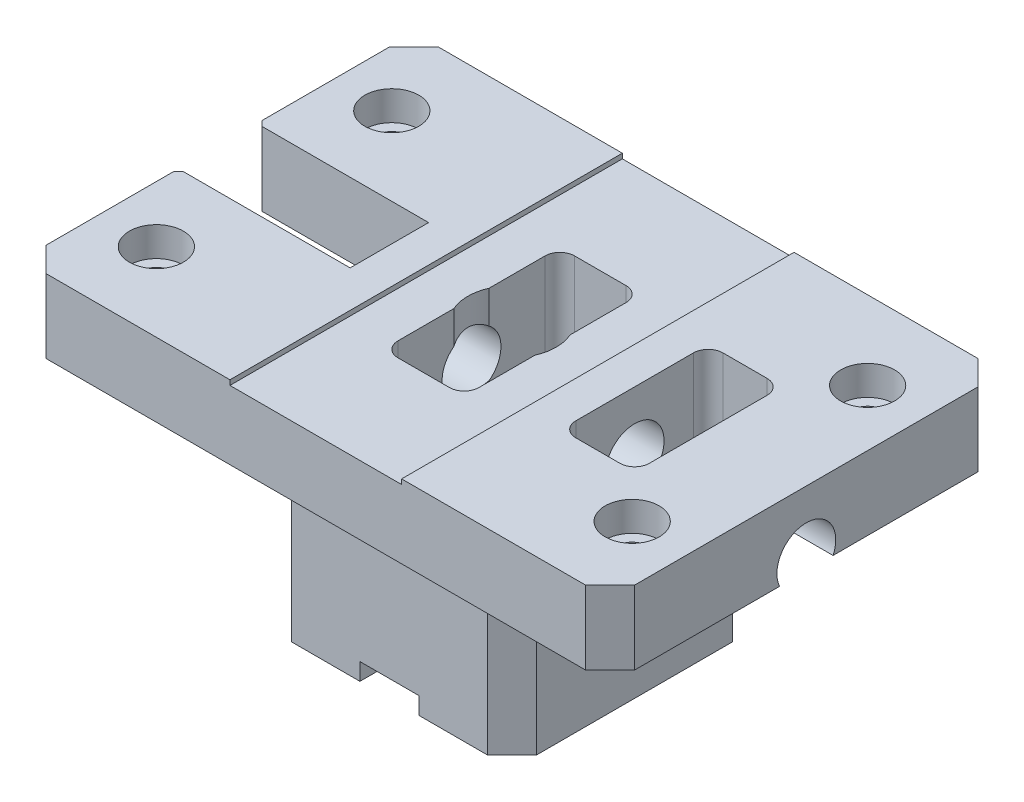
SolidWorks part; units mm, degrees
ref_plane "Front Plane" through (0, 0, 0) normal (0, 0, 1) x (1, 0, 0)
ref_plane "Top Plane" through (0, 0, 0) normal (0, 1, 0) x (1, 0, 0)
ref_plane "Right Plane" through (0, 0, 0) normal (1, 0, 0) x (0, 0, -1)
sketch "Sketch1" plane through (0, 0, 0) normal (0, 1, 0) x (1, 0, 0)
  line L1 (-60, 40) -> (60, 40)
  line L2 (-60, 40) -> (-60, -40)
  line L3 (-60, -40) -> (60, -40)
  line L4 (60, 40) -> (60, -40)
  line L5 (-60, 40) -> (60, -40) construction
  line L6 (-60, -40) -> (60, 40) construction
  point P0 (0, 0)
  dimension "D1" = 120
  dimension "D2" = 80
extrude "Boss-Extrude1" add sketch "Sketch1" along normal blind 15
sketch "Sketch2" plane through (0, 0, 0) normal (0, -1, 0) x (1, 0, 0)
  line L1 (-25, 25) -> (25, 25)
  line L2 (-25, 25) -> (-25, -25)
  line L3 (-25, -25) -> (25, -25)
  line L4 (25, 25) -> (25, -25)
  line L5 (-25, 25) -> (25, -25) construction
  line L6 (-25, -25) -> (25, 25) construction
  point P0 (0, 0)
  dimension "D1" = 50
  dimension "D2" = 50
extrude "Boss-Extrude2" add sketch "Sketch2" along normal blind 40
sketch "Sketch4" plane through (0, 15, 0) normal (0, 1, 0) x (1, 0, 0)
  line L1 (-5.25, 18) -> (5.25, 18)
  line L2 (-8.25, 15) -> (-8.25, -15)
  line L3 (-5.25, -18) -> (5.25, -18)
  line L4 (8.25, 15) -> (8.25, -15)
  line L5 (-8.25, 18) -> (8.25, -18) construction
  line L6 (-8.25, -18) -> (8.25, 18) construction
  arc A0 (-8.25, -15) -> (-5.25, -18) centre (-5.25, -15) ccw
  arc A1 (5.25, -18) -> (8.25, -15) centre (5.25, -15) ccw
  arc A2 (5.25, 18) -> (8.25, 15) centre (5.25, 15) cw
  arc A3 (-5.25, 18) -> (-8.25, 15) centre (-5.25, 15) ccw
  point P0 (0, 0)
  dimension "D3" = 3
  dimension "D1" = 16.5
  dimension "D2" = 36
extrude "Cut-Extrude2" cut sketch "Sketch4" against normal blind 33
sketch "Sketch5" plane through (-60, 0, 0) normal (-1, 0, 0) x (0, 0, 1)
  line L1 (-8, 20.6201) -> (8, 20.6201)
  line L2 (-8, 20.6201) -> (-8, -20.6201)
  line L3 (-8, -20.6201) -> (8, -20.6201)
  line L4 (8, 20.6201) -> (8, -20.6201)
  line L5 (-8, 20.6201) -> (8, -20.6201) construction
  line L6 (-8, -20.6201) -> (8, 20.6201) construction
  point P0 (0, 0)
  dimension "D1" = 16
  dimension "D2" = 41.2401
extrude "Cut-Extrude3" cut sketch "Sketch5" against normal blind 35
sketch "Sketch6" plane through (-25, 0, 0) normal (-1, 0, 0) x (0, 0, 1)
  line L0 (-8, 15) -> (8, 15) construction
  circle A0 centre (0, 2.5) radius 6
  dimension "D1" = 12
  dimension "D2" = 12.5
extrude "Cut-Extrude4" cut sketch "Sketch6" against normal through all
hole_wizard "CBORE for M6 Hex Socket Head Cap Screw1" positions "Sketch10" profile "Sketch9" counterbore size "M6" standard "ISO" end condition through all
sketch "Sketch10" plane through (0, 15, 0) normal (0, 1, 0) x (-1, 0, 0)
  line L0 (0, -40) -> (0, 40) construction
  line L1 (-60, -40) -> (60, -40) construction
  line L2 (60, 40) -> (-60, 40) construction
  line L4 (25, 0) -> (-31.5815, 0) construction
  line L5 (25, -8) -> (25, 8) construction
  point P1 (48.5, 24)
  point P3 (-48.5, 24)
  point P5 (-48.5, -24)
  point P7 (48.5, -24)
  dimension "D1" = 48
  dimension "D2" = 97
sketch "Sketch9" plane through (-48.5, 15, 24) normal (1, 0, 0) x (0, 0, 1)
  line L0 (0, 0) -> (0, 55)
  line L1 (0, 55) -> (3.3, 55)
  line L3 (3.3, 55) -> (3.3, 6)
  line L4 (3.3, 6) -> (5.5, 6)
  line L5 (5.5, 6) -> (5.5, 0)
  line L7 (5.5, 0) -> (0, 0)
  line L11 (0, -6.35) -> (0, 107.95) construction
  dimension "通孔孔直径" = 6.6
  dimension "通孔孔深度" = 55
  dimension "柱形沉头孔直径" = 11
  dimension "柱形沉头孔深度" = 6
sketch "Sketch11" plane through (0, -40, 0) normal (0, -1, 0) x (1, 0, 0)
  line L1 (-6, 30) -> (6, 30)
  line L2 (-6, 30) -> (-6, -30)
  line L3 (-6, -30) -> (6, -30)
  line L4 (6, 30) -> (6, -30)
  line L5 (-6, 30) -> (6, -30) construction
  line L6 (-6, -30) -> (6, 30) construction
  point P0 (0, 0)
  dimension "D1" = 12
  dimension "D2" = 60
extrude "Cut-Extrude5" cut sketch "Sketch11" against normal blind 3.5
sketch "Sketch13" plane through (0, 15, 0) normal (0, 1, 0) x (1, 0, 0)
  line L0 (60, -40) -> (60, 40) construction
  line L1 (28, 15) -> (37, 15)
  line L2 (25, 12) -> (25, -12)
  line L3 (28, -15) -> (37, -15)
  line L4 (40, 12) -> (40, -12)
  line L5 (0, 0) -> (68.6157, 0) construction
  arc A0 (37, 15) -> (40, 12) centre (37, 12) cw
  arc A1 (37, -15) -> (40, -12) centre (37, -12) ccw
  arc A2 (25, -12) -> (28, -15) centre (28, -12) ccw
  arc A3 (28, 15) -> (25, 12) centre (28, 12) ccw
  point P11 (40, 15)
  point P18 (25, 15)
  dimension "D4" = 3
  dimension "D1" = 15
  dimension "D2" = 35
  dimension "D3" = 30
extrude "Cut-Extrude7" cut sketch "Sketch13" against normal through all
chamfer "Chamfer1" distance 5 angle 45 8 edges at (60, 7.5, 40) (60, 7.5, -40) (-60, 7.5, -40) (-60, 7.5, 40) (25, -20, -25) (25, -20, 25) (-25, -20, 25) (-25, -20, -25)
chamfer "Chamfer2" distance 1 angle 45 2 edges at (-60, 7.5, 8) (-60, 7.5, -8)
sketch "Sketch14" plane through (0, 15, 0) normal (0, 1, 0) x (1, 0, 0)
  line L0 (-55, -40) -> (55, -40) construction
  line L1 (-17.5, 40) -> (17.5, 40)
  line L2 (-17.5, 40) -> (-17.5, -40)
  line L3 (-17.5, -40) -> (17.5, -40)
  line L4 (17.5, 40) -> (17.5, -40)
  line L5 (-17.5, 40) -> (17.5, -40) construction
  line L6 (-17.5, -40) -> (17.5, 40) construction
  point P0 (0, 0)
  dimension "D1" = 35
extrude "Cut-Extrude8" cut sketch "Sketch14" against normal blind 1
hole_wizard "CBORE for M10 Hex Socket Head Cap Screw1" positions "Sketch8" profile "Sketch7" counterbore size "M10" standard "ISO" end condition through all
sketch "Sketch8" plane through (-12.6368, 14, 0.8834) normal (0, 1, 0) x (-1, 0, 0)
  point P0 (-12.6368, -0.8834)
sketch "Sketch7" plane through (0, 14, 0) normal (1, 0, 0) x (0, 0, 1)
  line L0 (0, 0) -> (0, 54)
  line L1 (0, 54) -> (5.5, 54)
  line L3 (5.5, 54) -> (5.5, 42)
  line L4 (5.5, 42) -> (9, 42)
  line L5 (9, 42) -> (9, 0)
  line L7 (9, 0) -> (0, 0)
  line L11 (0, -6.35) -> (0, 107.95) construction
  dimension "通孔孔直径" = 11
  dimension "通孔孔深度" = 54
  dimension "柱形沉头孔直径" = 18
  dimension "柱形沉头孔深度" = 42
